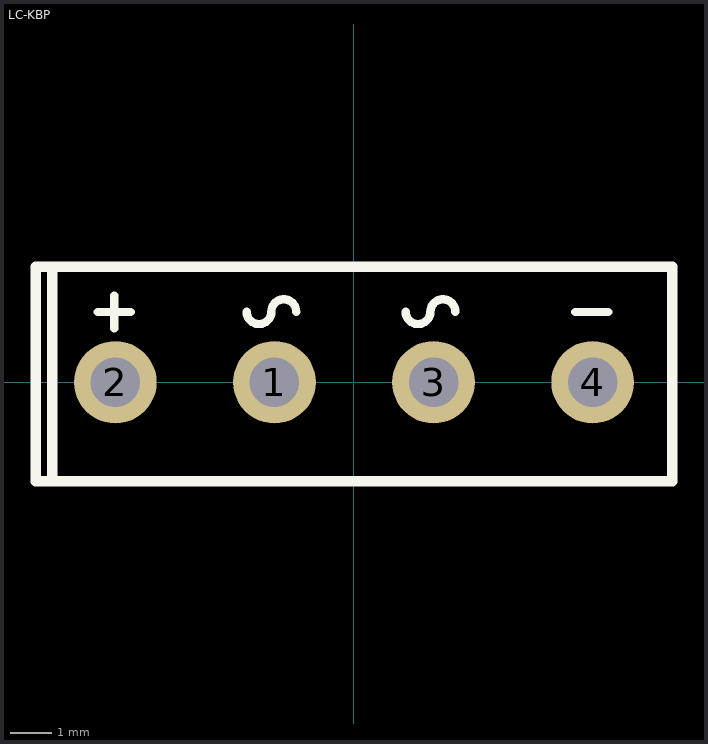
[diagram p0: the footprint, top view; thin cyan lines are the x and y axes]
# Altium footprint library MISC89340-22.PcbLib: 1 footprints
Each footprint in its own frame and in the unit in brackets; x right, y up, seen from the top. Pads: shape width x height; smd on the part's side, far side on the other; paste and mask are expansions set on the pad; w line width, h text height; cw(c..) or ccw(c..) is an arc to the next point about the centre after c.

## LC-KBP [mm]
pads (4):
  round 2 hole 1.2: 1(-1.925,0) 2(-5.775,0) 3(1.925,0) 4(5.775,0)
Top Overlay:
  lines w0.203: -6.2,1.7 -5.4,1.7 ; -5.8,1.3 -5.8,2.1 ; -2.6,1.708 ccw(c-2.3,1.708) -2,1.708 cw(c-1.7,1.708) -1.4,1.708 ; 1.25,1.708 ccw(c1.55,1.708) 1.85,1.708 cw(c2.15,1.708) 2.45,1.708 ; 5.35,1.7 6.15,1.7
  lines w0.254: -7.3,-2.4 -7.3,2.8 ; -7.7,-2.4 -7.7,2.8 7.7,2.8 7.7,-2.4 -7.7,-2.4